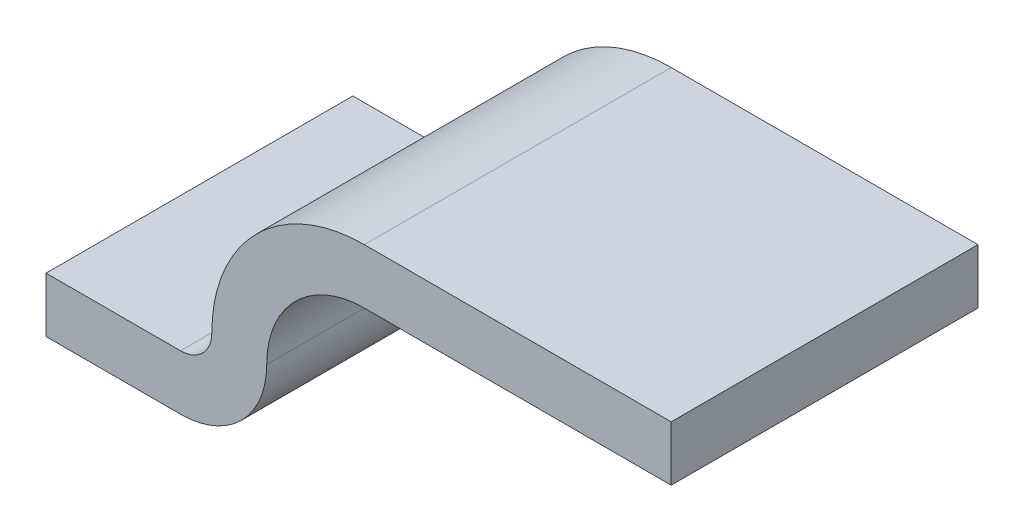
from build123d import *

# Parameters (mm, degrees)
BOSS_EXTRUDE1_DEPTH = 22.352


with BuildPart() as part:
    # Sketch1 → Boss-Extrude1 (new body)
    with BuildSketch(Plane.XY):
        with BuildLine():
            Line((0, 11.112), (22.35, 11.112))
            Line((22.35, 11.112), (22.35, 7.112))
            Line((22.35, 7.112), (0, 7.112))
            ThreePointArc((0, 7.112), (-5.028943428, 5.028943428), (-7.112, 0))
            ThreePointArc((-7.112, 0), (-8.951369414, -4.440630586), (-13.392, -6.28))
            Line((-13.392, -6.28), (-23.192, -6.28))
            Line((-23.192, -6.28), (-23.192, -2.28))
            Line((-23.192, -2.28), (-13.392, -2.28))
            ThreePointArc((-13.392, -2.28), (-11.779796539, -1.612203461), (-11.112, 0))
            ThreePointArc((-11.112, 0), (-7.857370553, 7.857370553), (0, 11.112))
        make_face()
    extrude(amount=BOSS_EXTRUDE1_DEPTH)


solid = part.part
